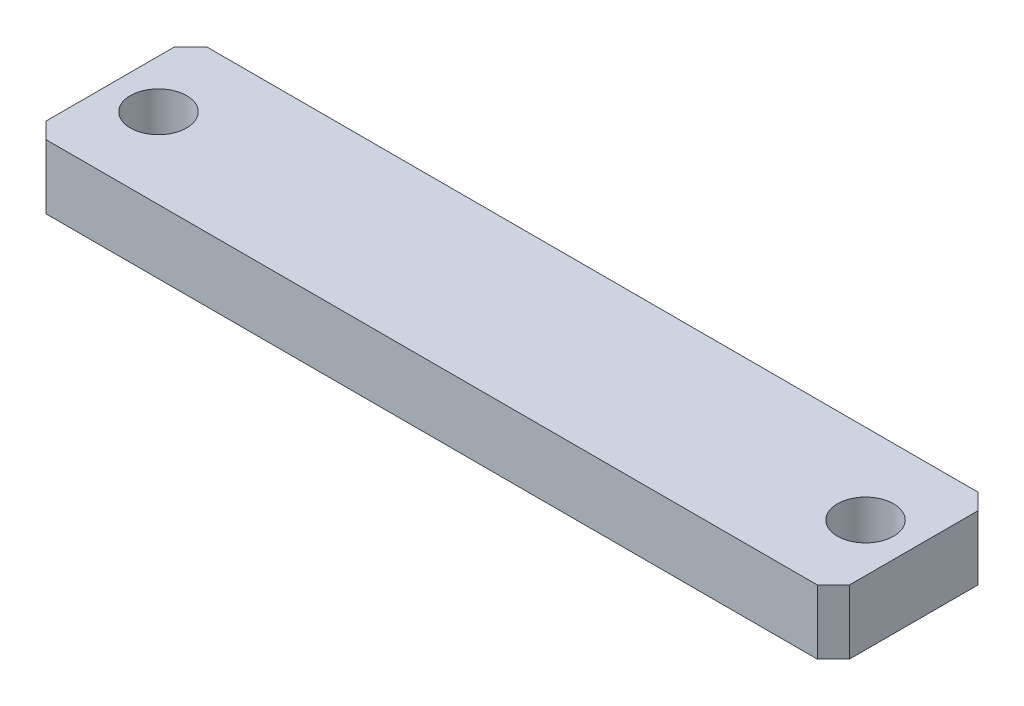
from build123d import *

# Parameters (mm, degrees)
SKETCH1_W                  = 50
SKETCH1_H                  = 10
BOSS_EXTRUDE1_DEPTH        = 2
F_3_5_3_5_DIAMETER_HOLE1_D = 3.5
CHAMFER1_SIZE              = 1
CUT_EXTRUDE1_DEPTH         = 2


with BuildPart() as part:
    # Sketch1 → Boss-Extrude1 (new, symmetric)
    with BuildSketch(Plane(origin=(0, 0, 0), x_dir=(1, 0, 0), z_dir=(0, 1, 0))):
        Rectangle(SKETCH1_W, SKETCH1_H)
    extrude(amount=BOSS_EXTRUDE1_DEPTH, both=True)

    # Ø3.5 (3.5) Diameter Hole1 (through all)
    with Locations(Plane(origin=(0, 2, 0), x_dir=(1, 0, 0), z_dir=(0, 1, 0))):
        with Locations((-22, 0), (22, 0)):
            Hole(F_3_5_3_5_DIAMETER_HOLE1_D / 2)

    # Chamfer1
    chamfer1_edges = [part.edges().sort_by_distance(p)[0] for p in [
        (25, 0, 5),
        (-25, 0, 5),
        (-25, 0, -5),
        (25, 0, -5),
    ]]
    chamfer(chamfer1_edges, length=CHAMFER1_SIZE)

    # Sketch4 → Cut-Extrude1 (cut)
    with BuildSketch(Plane.XZ.offset(2)):
        with BuildLine():
            Line((-17, 3.5), (17, 3.5))
            ThreePointArc((17, 3.5), (18.414213562, 2.914213562), (19, 1.5))
            Line((19, 1.5), (19, -1.5))
            ThreePointArc((19, -1.5), (18.414213562, -2.914213562), (17, -3.5))
            Line((17, -3.5), (-17, -3.5))
            ThreePointArc((-17, -3.5), (-18.414213562, -2.914213562), (-19, -1.5))
            Line((-19, -1.5), (-19, 1.5))
            ThreePointArc((-19, 1.5), (-18.414213562, 2.914213562), (-17, 3.5))
        make_face()
    extrude(amount=-CUT_EXTRUDE1_DEPTH, mode=Mode.SUBTRACT)


solid = part.part
